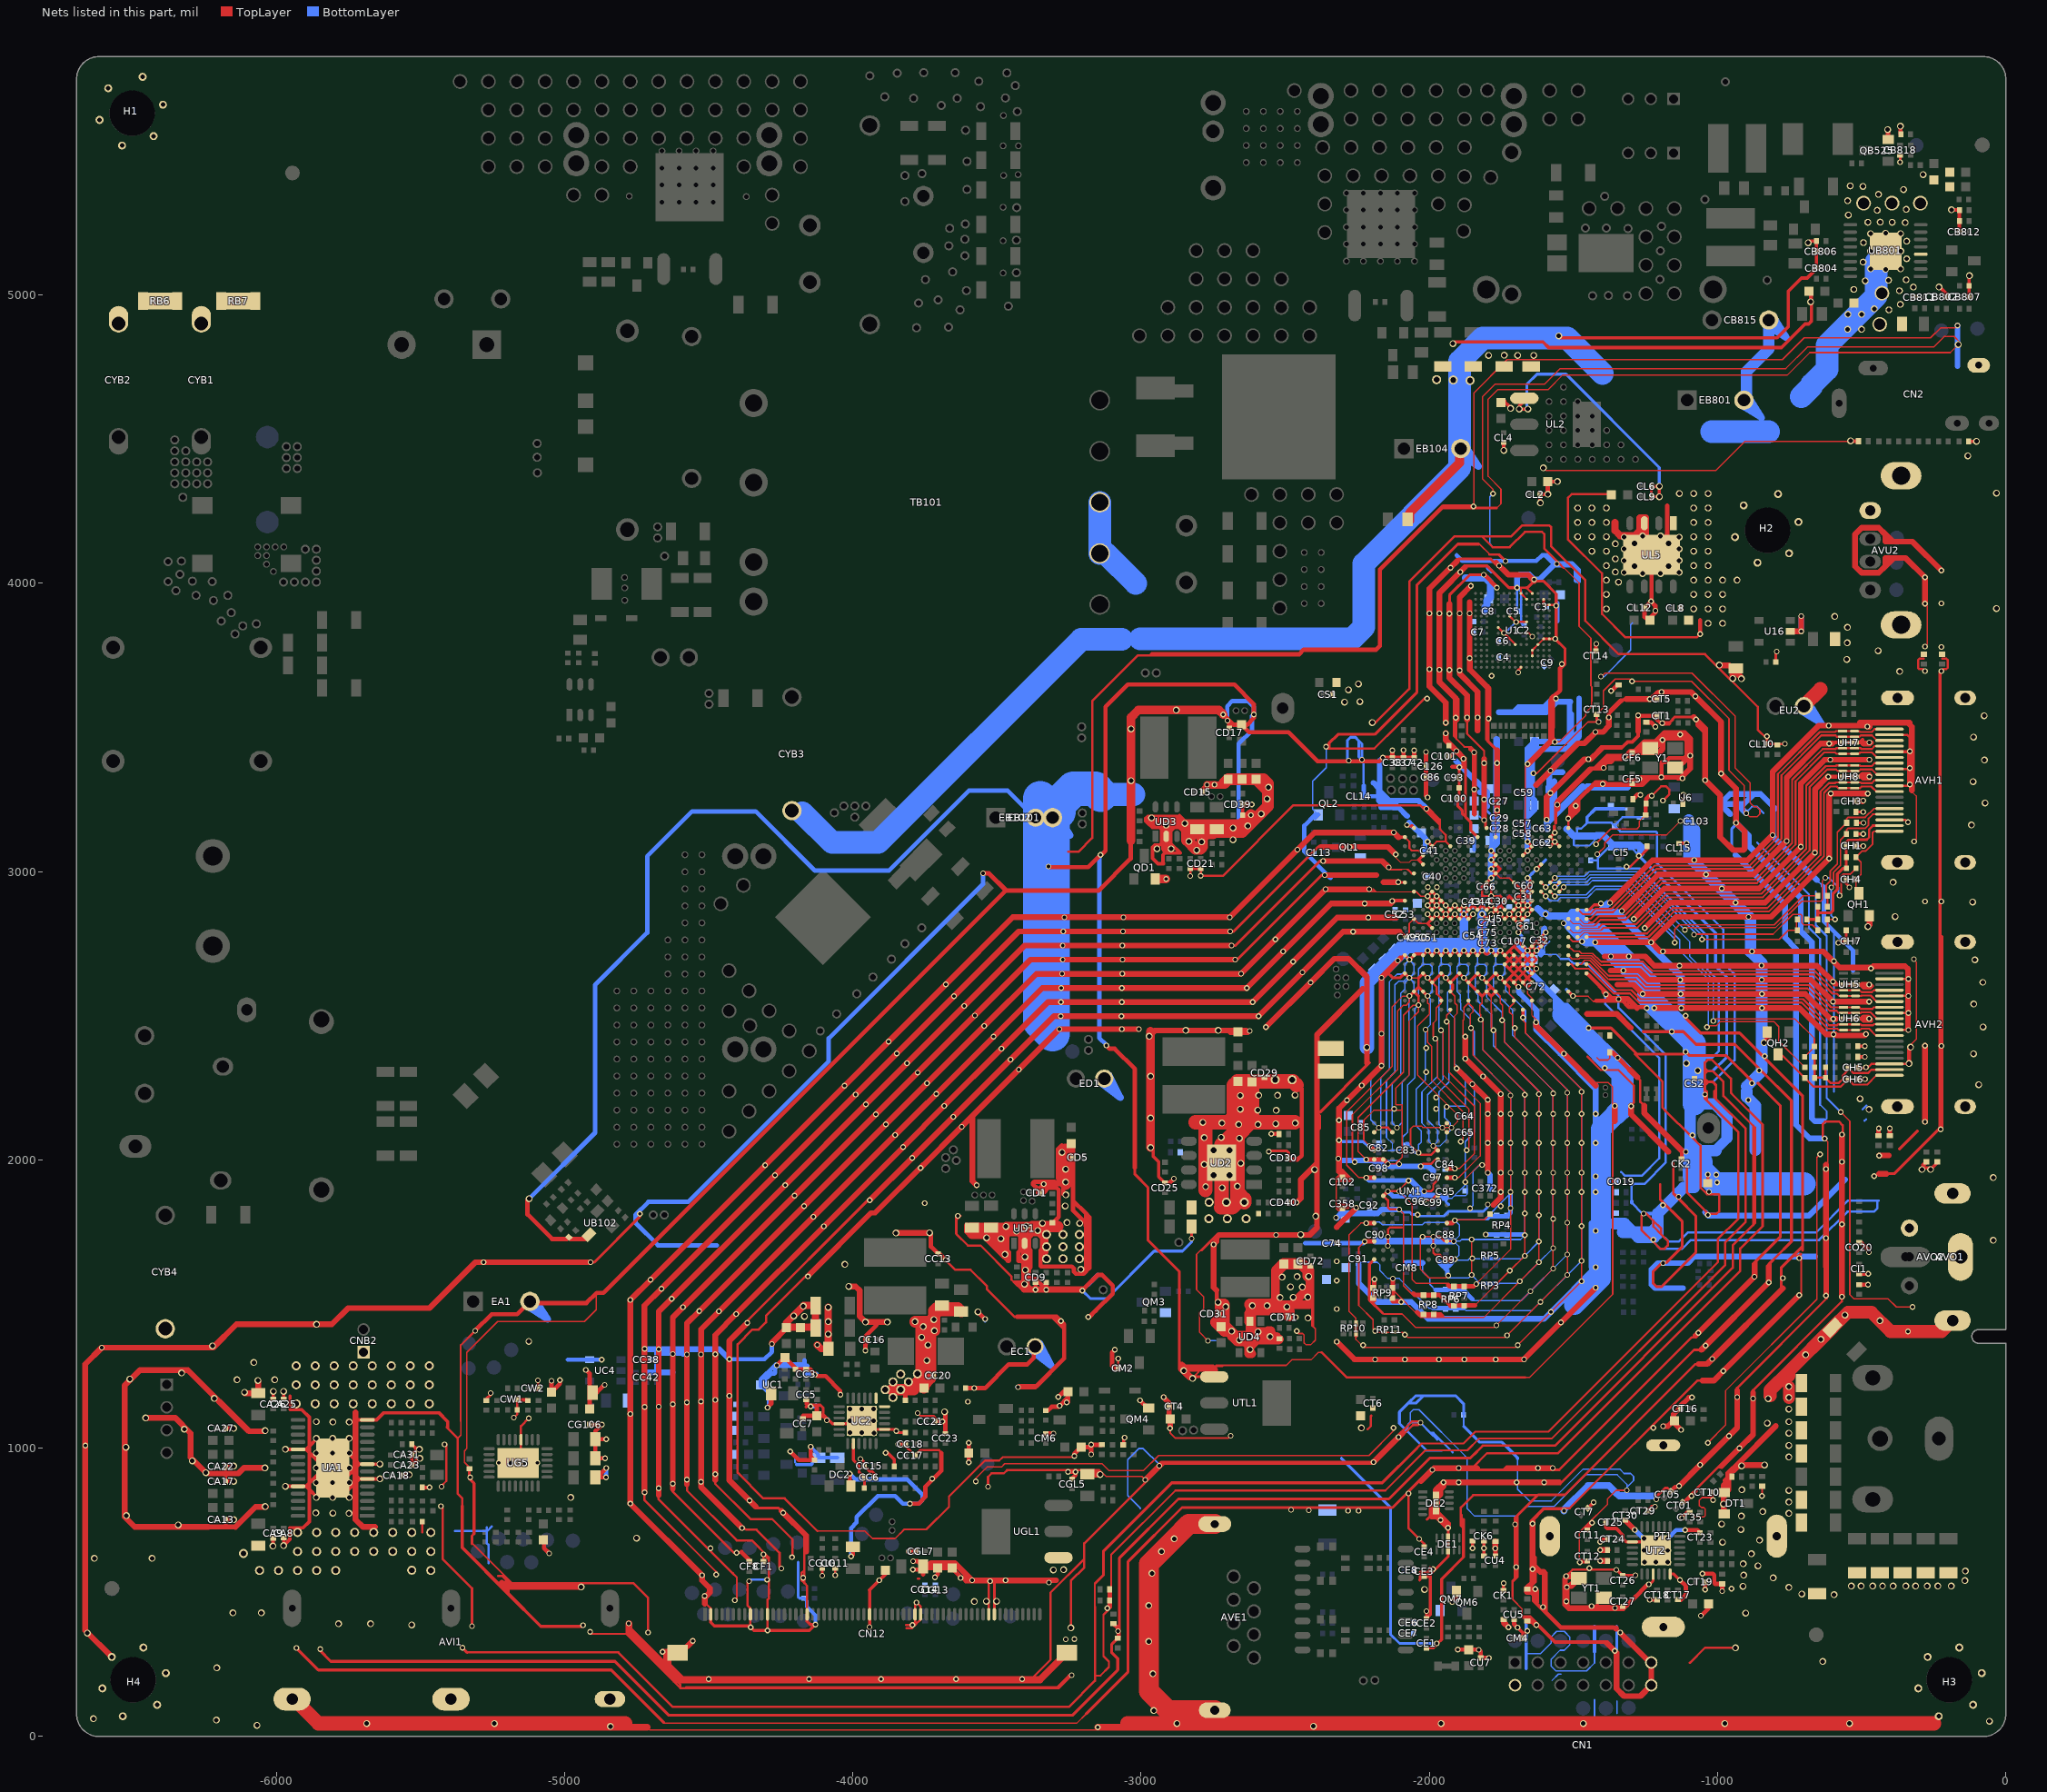
[diagram p0: the nets of this part, all layers, seen from the top]
# Altium PCB MISC84395.PcbDoc (part 19 of 26)
Units mil, origin at the board's own origin, x right, y up, seen from the top; angles counter-clockwise.
Board outline 6692.91 x 5826.77 mil, 2 copper layers (TopLayer, BottomLayer), stack 61.855 mil thick; 951 components, 565 nets, 4374 pads, 1804 vias.
Unrouted connection lines stored in the file: 1.

## Via types
v1: diameter 19.68, hole 11.81, TopLayer to BottomLayer, tented both sides, 1262 vias
v2: diameter 23.62, hole 15.75, TopLayer to BottomLayer, tented both sides, 524 vias
v3: diameter 31.5, hole 19.68, TopLayer to BottomLayer, tented both sides, 11 vias
v4: diameter 24, hole 16, TopLayer to BottomLayer, tented both sides, 6 vias
v5: diameter 19, hole 11.81, TopLayer to BottomLayer, tented both sides, 1 vias

## Nets (pads, with @x,y where several pads share a name; then routed paths per layer and width w, separated by ;. In a path a pad name is that pad's centre, name@x,y a point inside that pad or via, vN(x,y) a via of type N, cw(c..) or ccw(c..) an arc to the next point about the centre after c; other vN are vias at no path point) (continued)
GND: (continued)
  BottomLayer w20: v1@-4722.5,1343 v1(-4673.5,1343) -4463,1343 v1(-4428.5,1308.5) ; CC42.2@-4716,1262.46 RC31.1@-4679,1262.46 ; -4624.46,1262.46 RC31.1@-4679,1262.46 ; -4589,1328 -4591,1330 -4679,1330 RC31.1@-4679,1262.46 ; v1(-1908.55,3533.74) -1908.55,3531.89 v1@-1906.65,3529.99 ; -1906.65,3382.47 -1881.15,3356.97 C26.1@-1799.15,3274.97 ; -1824.78,3274.97 -1806.22,3274.97 C26.1@-1799.15,3274.97 ; -1799.15,3226.74 C26.1@-1799.15,3274.97 ; -1759.65,3552.74 -1707.65,3552.74 ; v1(-1695.65,3984.74) -1695.65,4019.87 -1685.78,4029.74 -1653.65,4029.74 v1(-1636.65,4012.74) -1618.65,4012.74 -1566.35,4065.04 v1@-1564.15,4067.24 ; -1689.7,2743.77 -1683.77,2743.77 -1665.85,2725.85 -1655.42,2715.42 -1655.42,2697.07 -1662.66,2689.82 -1662.66,2664.62 -1608.01,2609.96 -1608.01,2607.83 ; -1653.08,3196.76 -1636.19,3213.65 C55.1@-1636.19,3231 -1636.19,3248.35 -1644.08,3256.24 -1644.08,3405.63 ; v1@-1633.27,510.73 v1(-1633,511) ; v1(-1628.24,2725.85) -1627.69,2725.85 -1616.72,2736.82 ; C72.1@-1621.58,2621.07 -1561.83,2561.32 ; -1613.82,2712.88 -1606.49,2720.21 ; -1603.39,2777.66 -1603.39,2799.74 -1600.39,2802.74 ; v1@-1589.5,3184.5 -1576.82,3197.18 -1576.82,3264.82 -1588,3276 -1588,3292.28 -1583.87,3296.41 ; -1580.65,3591.74 -1602.65,3569.74 -1690.65,3569.74 -1707.65,3552.74 ; -1567,3216 -1567,3313.28 -1583.87,3296.41 ; -1538.01,3344.95 -1571.15,3344.95 -1571.89,3345.69 -1583.87,3345.69 -1583.87,3296.41 ; -1510.65,3588.74 -1558.07,3588.74 -1594.07,3552.74 -1707.65,3552.74 ; -1119.84,1555.16 -1216.48,1555.16 -1228.84,1567.52 -1228.84,1620.16 -1207.2,1641.8 v1(-1189,1641.8) -1103.96,1641.8 -1080.76,1665 -662,1665 ; -1043.29,1818.5 -1031.94,1807.16 -683.22,1807.16 -558.44,1931.94 ; -955.99,3199 -990.99,3234 ; -938.62,3058.12 -766.46,2885.96 -766.46,2770.58 -728,2732.12 -728,2121.5 -680.63,2074.13 v1(-629,2074.13) ; v1(-935.99,3169.07) -891.31,3124.39 -891.31,3088.59 -711.46,2908.74 -711.46,2793.36 -673,2754.91 -673,2144.28 -662.85,2134.13 -631.13,2134.13 ; v1(-900.83,3202) -932.83,3234 ; -799.83,3218 -808.31,3226.47 ; v1@-719.46,1665.47 v1@-716.84,1668.09 ; v1(-709.84,3833) v1(-709.84,3886) ; -655.59,2970.25 -808.31,3122.97 -808.31,3226.47 ; -168,4753 -168,4864 ; v2@-168,4831 -168,4864 ; v1(-168,4894) -168,4864 ; -1561.83,2561.32 -1535.09,2534.57 -1522.81,2534.57 -1446.73,2458.49 -1490.24,2458.49 -1494.67,2458.49 C106.1@-1539.5,2503.33 -1561.83,2525.66 -1561.83,2561.32 ; -990.99,3234 -956.15,3268.84 -874.12,3268.84 ; -990.99,3234 -932.83,3234 ; -932.83,3234 -908.97,3234 -874.12,3268.84 ; -874.12,3268.84 -850.68,3268.84 -808.31,3226.47
  BottomLayer w23.62: EB101.2@-3307.15,3187 -3305.99,3187 -3267,3225.99 ; C90.1@-2187.29,1717.65 -2187.29,1717.97 v1(-1915.64,1717.97)
  BottomLayer w24: v1(-1785.72,2977.82) v1(-1785.72,3009.31) v1(-1785.72,3040.81) -1785.72,3045.21 -1782.21,3048.72 -1782.21,3051.5 -1781.97,3051.74 -1781.97,3084.13 -1766.47,3099.63 -1766.47,3151.31 -1766.47,3458.56 ; v1(-1533,783) -1533,787 -1449,871 -1378.04,871 -1353.02,845.98 -1341.04,834 -1222,834
  BottomLayer w25: -1875.35,4018.03 -1805.34,4018.03 -1788.17,4000.86 -1788.17,3952.03 C108.1@-1794.46,3945.74 -1800.98,3939.22 -1800.98,3923.3 -1807.74,3916.54 C8.1@-1807.74,3902.74 ; -1623.84,2871.76 -1607.82,2855.74 -1597.44,2855.74 -1587.09,2845.4 -1517.69,2845.4 -1503.69,2859.4 -1410.7,2859.4 ; C63.1@-1592.83,3147.83 C63.1@-1590.92,3149.74 -1590.91,3171.47 -1468.65,3293.74 ; -1522.65,3147.74 -1497.65,3122.74 -1487.65,3122.74 -1422.26,3122.74 -1419.31,3125.69 -1396.66,3125.69 -1363.37,3092.4 ; -1451.65,3293.74 -1313.7,3293.74 ; v1@-1381.15,2888.96 -1410.7,2859.4 ; -1353.18,3082.2 -1353.45,3082.47 -1363.37,3092.4 ; -1266.15,3062.36 -1266.15,3086.01 -1272.54,3092.4 -1363.37,3092.4 ; v1(-1125.83,2526.9) -1125.83,2635.24 -1349.99,2859.4 -1410.7,2859.4
  BottomLayer w30: -1880.2,2745.28 v1(-1880.2,2851.83) ; -1824.76,2744.72 -1818.59,2750.9 C75.1@-1818.59,2792.52 ; v1(-1817.21,2851.83) -1818.59,2850.45 -1818.59,2837.74 ; -1798.22,2724.06 -1813.78,2739.62 -1813.78,2787.71 C75.1@-1818.59,2792.52 ; -1634.71,3404.04 C56.1@-1634.71,3451.34 ; C75.1@-1818.59,2792.52 -1818.59,2809.09 ; -1818.59,2809.09 -1818.59,2837.74 ; -1818.59,2809.09 -1808.77,2818.91 -1808.77,2827.92 -1818.59,2837.74
  BottomLayer w34: -1005.86,2031.95 -1005.86,2035.75 -967.92,2073.68 -967.92,2076.65
  BottomLayer w39.37: -1096.03,2023.03 -1096.03,2179.24 -1080.8,2194.47 -1011.88,2194.47 -967.92,2150.51 -967.92,2076.65 ; -1057,2031.95 -1005.86,2031.95 ; EB801.2@-899.5,4644.3 -899.5,4735 -822.57,4811.93 -822.57,4850.5 ; -822.57,4826 -822.57,4850.5 ; CB815.2@-822.57,4912 -822.57,4850.5
  BottomLayer w40: -1359,1779 -1322.96,1779 -1293.11,1749.16 ; -1329.16,1749.16 -1293.11,1749.16 ; -1099.8,3178.58 -1099.8,3156.65 ; -1093.84,3157.16 -1080.32,3143.65 -1080.32,3137.17 ; -1080.8,1943.9 -1080.8,1904 -1118.32,1904 -1208,1814.32 -1208,1786.27 ; v1@-1080.32,3045.67 -1080.32,3137.17 ; -899,2238.1 -899,2218.32 -869,2188.32 -869,2034 ; -899,2255.1 -847.3,2306.79 -847.3,2683.14 -885.46,2721.29 -885.46,2836.67 -1099.8,3051.01 -1099.8,3156.65 ; -1293.11,1749.16 -1275.96,1732 v1@-1223.48,1732 ; -1293.11,1749.16 -1230.57,1749.16 -1208,1771.73 -1208,1786.27 ; v1@-1223.48,1732 -1207.16,1748.32 ; v1@-1223.48,1732 -1220.27,1732 -1207.16,1745.12 -1207.16,1748.32 ; -1208,1786.27 -1207.16,1785.43 -1207.16,1748.32 ; -1099.8,3156.65 -1080.32,3137.17
  BottomLayer w50: v2(-2216.77,2390.46) -2216.77,2614.62 -2216.65,2614.74 -2087.26,2744.12 -2062.3,2744.12 -2061.7,2744.72 -1824.76,2744.72
  BottomLayer w70: -1497,1497 -1404.83,1589.17 -1404.83,1776.93 -1404.83,2107 -1351.83,2160
  BottomLayer w76: C106.1@-1535.33,2506 -1535.33,2503.58 -1490.24,2458.49 -1330.18,2298.42 -1330.18,2181.66 -1351.83,2160
  BottomLayer w78.74: -4175,3204 -4072,3101 -3912,3101 -3208,3805 -3067,3805 ; TB101.9@-3143.53,4280.51 TB101.8@-3143.53,4103.35 -3122.35,4103.35 -3018,3999 ; -3003,3807 -2268,3807 -2227,3848 -2227,4068 -1895.57,4399.43 -1895.57,4446.85 -1895.57,4769.43 -1815,4850 -1615,4850 -1522,4850 -1399.5,4727.5 ; -1020,4526 -823,4526 ; -710,4647 -673.7,4683.3 -673.7,4688.94 -620.87,4741.76 -620.87,4825.41 -450,4996.28 -450,5114
  BottomLayer w80: -3267,3225.99 -3225.99,3267 -3139.72,3267 -3025,3267 ; -1495.52,2824.48 -1451.55,2780.51 -1413.62,2780.51 -1238.8,2605.69 -1238.8,2562.55 -1080.8,2404.55 -1080.8,2194.47 ; -1080.8,2023.03 -1080.8,1943.9 -1075.9,1939 ; -1056.84,1992.41 -1056.84,1966.28 -1008.06,1917.5 -699.5,1917.5
  BottomLayer w120: -3350,3254 -3350,2478.91 -3307.15,2436.06 -3307.15,3164.02 EB101.2@-3307.15,3187 -3287,3207.15 -3287,3234.28 -3234.28,3287 -3159.72,3287 -3139.72,3267
  other v1: -1356.73,296.85 -1828.62,300.62 -5847,303 -3261.5,337 -3231.5,338 -4296,367.66 -1356,446 -1606,449 -4514,488 -3320,534 -4297.18,544 -4172,551 -1351.29,578.23 -1987.32,580.62 -1699,588 -1407,647 -4494,653 -2035.21,685.57 -1436,741 -2282,783 -2246,783 -2418,785 -2480,786 -1090.4,834.5 -1602,882 -3573.71,884.84 -5327,899 -1623.5,931 -5228,949 -5094,949 -5416.23,1013 -960.45,1042.47 -1223,1071 -3601,1161 -4263.22,1287.7 -2188.27,1308.03 -2084.93,1308.03 -1966.82,1308.03 -1878.24,1308.03 -1769.97,1308.03 -1041.72,1355.98 -2230.11,1357.25 -1693.69,1357.25 -340,1405 -2188.27,1406.46 -1543.59,1435.99 -4464.4,1475.03 -2321.15,1482.74 -4588.71,1489.31 -4628.72,1518.59 -624,1529 -2321.15,1581.16 -774,1590 -2321.15,1648.26 -1850.76,1658.41 -717,1659 -1986.51,1702.22 -2143.99,1733.72 -1423.02,1753.92 -1472.23,1770.56 -1521.45,1782.51 -1570.66,1795.33 -2323.62,1799.76 -1619.87,1807.86 -1034,1809 -1669.08,1814.64 -1718.3,1832.36 -2253.99,1833.85 -1752.74,1839.53 -1190,1843 -1797.3,1844.91 -3751,1850 -4201.82,1876.2 -1752.74,1888.74 -1669.08,1888.74 -1619.87,1888.74 -1570.66,1888.74 -1521.44,1888.74 -1472.23,1888.74 -457,1944 -1004.41,1948.42 -1752.74,1955.18 -1718.29,1955.18 -1669.08,1955.18 -1619.87,1955.18 -1570.66,1955.18 -1521.44,1955.18 -1472.23,1955.18 -4304.17,1981.74 -2104.62,1985.69 -1110,2028 -1870.85,2033.92 -1797.03,2058.52 -1752.74,2058.52 -1718.29,2058.52 -1669.08,2058.52 -1619.87,2058.52 -1570.66,2058.52 -1521.44,2058.52 -1472.23,2058.52 -3853.06,2086.36 -3919.97,2158.05 -1797.03,2159.41 -1752.74,2159.41 -1718.29,2159.41 -1669.08,2159.41 -1619.87,2159.41 -1570.66,2159.41 -1521.44,2159.41 -1472.23,2159.41 -2121.84,2176.63 -1976.66,2176.63 -1939.75,2184.01 -2285.86,2207 -894,2208 -1976.66,2216 -1718.3,2223.38 -1669.08,2225.84 -1619.87,2228.31 -3710.48,2228.95 -1570.66,2230.77 -1472.23,2235.69 -2235.03,2257.83 -3775.38,2302.64 -2011.11,2304.58 -1346.8,2354.14 -837.15,2359.99 -2011.11,2388.25 -3512.01,2427.42 -2166.13,2437.46 -1159,2445 -2623,2447 -338.37,2450.71 -1856.09,2457.14 -3576.91,2501.11 -338.37,2509.76 -338.37,2568.82 -1128.65,2575.74 -600,2618 -1129.65,2624.74 -2440.45,2650.55 -1659.73,2662.86 -1132.65,2673.74 -2109.54,2691.39 -319,2696 -2506.97,2722.62 -1189.65,2722.74 -1597,2852 -281,2896 -223.83,2896 -2129.06,2897.57 -2116.65,3059.74 -2123.65,3135.74 -2077.58,3161.48 -1492.65,3227.74 -1272,3322 -333.37,3358.78 -2012,3415 -333.37,3416.78 -1794.65,3530.74 -1560.65,3599.74 -1784,3679 -1692.21,3690.34 -280.83,3695.5 -1540.65,3719.74 -223.83,3779 -1563.62,3807.03 -223.83,3930 -1892.65,4038.74 -1758.33,4061.24 -367,5460
  other v2: -4841,35 -2402,36 -6067,39 -57,53 -6208,57 -6634,62 -2956,90 -2959,218 -6206,238 -636,260 -6655,359 -5530,387 -5784,391 -5673,391 -903,428 -6150,429 -6052,429 -3578.5,468 -3536.5,469.5 -3501.5,469.5 -596,492 -708,494 -2017,510 -753,517 -912,521 -536,522 -502.57,522 -462.57,522 -428,522 -391,522 -347,522 -313,522 -273,522 -236,522 -190,522 -142,541 -807,550 -910,560 -2962,566 -141,574 -3304,578 -3269,579 -860,592 -911,599 -1254.34,604.53 -1213.81,604.28 -1172.92,604.41 -6631,618 -6431,618 -883,634 -1255.16,645.42 -1172.72,645.25 -983,674 -855,681 -1254.99,686.64 -1214.11,686.47 -4750,688 -919,718 -6340,734 -986,737 -918,765 -6520,766 -5747.94,774 -752.76,773.79 -5803.94,775 -5862.94,776 -844,780 -980,806 -752.76,813.79 -5861.24,829.58 -5804.15,829.58 -5747.07,829.58 -4979,829 -752.76,853.79 -916,856 -5861.24,880.76 -5804.15,880.76 -5747.07,880.76 -5861.24,931.94 -5747.07,931.94 -917,939 -5186,949 -5136,949 -6291,956 -5501.56,964.94 -752.76,969.79 -5861.24,983.12 -5804.15,983.12 -5747.07,983.12 -5503.27,996.65 -6521,1003 -752.76,1009.79 -5861.24,1034.3 -5804.15,1034.3 -5747.07,1034.3 -753,1052 -3968.66,1053.73 -3926.59,1053.07 -4009.8,1053.95 -6319,1066 -6148.23,1069 -2236,1070 -828,1087 -5803.94,1091 -5746.94,1091 -5860.94,1092 -753,1092 -4009.93,1094.84 -3927.55,1095 -4009.71,1135.98 -3968.82,1136.11 -3927.68,1135.89 -753,1136 -825,1172 -6214.94,1173 -753,1176 -6109.94,1194 -6063.94,1235 -6135.94,1237 -6004.94,1237 -6508,1240 -2821,1242 -6328,1261 -6077.94,1297 -3743,1304 -694.34,1323.66 -6221,1355 -3739,1358 -5124,1370.5 -2659,1375 -641.98,1377.53 -3761,1385 -2553,1387 -2594,1404 -2686,1406 -3755.57,1421.43 -437.43,1442.43 -3719,1446 -2421,1452 -4168,1457 -4205,1459 -558.35,1461.6 -2494,1490 -2706,1491 -4172,1493 -2614,1494.26 -2563,1494.26 -2733,1506 -2518,1522.26 -2472,1523 -2422,1524.26 -2441,1559 -2482,1560 -2511,1593.26 -2459,1595.26 -2419,1596.26 -3401,1618 -4028,1638 -44,1721 -2446,1741 -3432,1753 -3359,1755 -3469,1769 -3398,1771 -3342,1780 -3213,1780 -3257,1783 -2394,1805 -3263,1840 -3261,1879 -2719,1903 -2776,1907 -2666,1909 -44,1939 -2398,1966 -2781,1984 -2654,1988 -3274,2026 -2659,2075 -2781,2077 -2722,2078 -2661,2123 -2594,2123 -2533,2125 -2720,2128 -2465,2128 -2786,2130 -2531,2172 -2595,2173 -474.55,2175.28 -2656,2176 -506,2211.85 -2656,2223 -2592,2224 -2527,2224 -2466,2225 -94.37,2260.84 -1069,2309.51 -1108,2335 -112.37,2367.84 -79.37,2460.84 -111.37,2540.84 -80.37,2615.84 -107.37,2693.84 -384,2844 -115.37,2894.16 -391.36,2963.29 -2630,3158 -119.37,3161.16 -2583,3200 -72.37,3238.16 -2563,3252 -2558,3292 -114.37,3312.16 -74.37,3387.16 -112.37,3466.16 -75.37,3540.16 -2294,3588 -2241,3589 -2281,3630 -2246,3651 -368.29,3694 -551.83,3736 -443,3766 -550.83,3793 -549.83,3847 -32.5,3912.4 -1260.33,4033.47 -1198.07,4033.47 -1324.58,4037.62 -1133.83,4037.62 -1324.58,4078.24 -1133.83,4078.24 -1324.58,4118.86 -1133.83,4118.86 -1324.58,4159.47 -1133.83,4159.47 -1260.33,4163.62 -1198.08,4163.62 -32.5,4313 -132,4442 -1742,4461 -417.58,5088.39 -469.55,5090.37 -365.61,5090.37 -470.33,5151.39 -364.82,5151.39 -469.55,5212.42 -365.61,5212.42 -417.58,5214.39 -287,5417
  other v3: -2748.56,1946.69 -2693.44,1946.69 -2748.56,2033.31 -2693.44,2033.31 -1288.26,4059.18 -1170.15,4059.18 -1288.27,4137.92 -1170.15,4137.92
  other v5: -1837.35,1569.72
GVOFF: CC6.2 RC6.1 UC2.8 | length 169.9
  TopLayer w10: UC2.8@-3998.27,1016.18 -3998.27,959.21 -3978.59,939.53 -3978.59,917.7 CC6.2@-3959.89,899 ; RC6.1@-3959.73,862 CC6.2@-3959.73,898.84
HDMI1_5V: AVH1.18 CH1.1 RH1.1 RH2.1 RH4.1 RH5.1 RH8.1 | length 594
  TopLayer w6: -546.2,3109.96 -545.7,3110.46
  TopLayer w8: -545.7,3110.46 -507.06,3110.46 -506.87,3110.65 -483.02,3110.65 -474.38,3119.29 -474.38,3146.59 -461.51,3159.45 AVH1.18@-403.84,3159.45
  TopLayer w10: RH2.1@-693.1,2834 RH5.1@-652.57,2834 -652.57,2857 ; RH4.1@-652.57,2878 -652.57,2857 ; -545.7,3109.46 -553.57,3101.6 RH1.1@-553.57,3050 RH8.1@-553.57,3011 -566.06,3011 -584.83,2992.22 -584.83,2937.99 -600.24,2922.58 -600.24,2864.01 -607.26,2857 -652.57,2857
HDMI1_CLKN_IC: AVH1.12 U5.J1 UH8.4 UH8.5 | length 1408.2
  TopLayer w7: U5.J1@-1455.01,2773.09 -1454.67,2773.43 -1239.8,2773.43 -1151.95,2861.28 -822.88,2861.28 -631.33,3052.83 -631.33,3272.66 -608.87,3295.12 -587.37,3295.12 -581.66,3289.41 UH8.4@-565.81,3289.41 UH8.5@-524.87,3289.41 -506.09,3289.41 -500.37,3295.12 -467.12,3295.12 -449.56,3277.56 AVH1.12@-403.84,3277.56
HDMI1_CLKP_IC: AVH1.10 U5.J2 UH8.3 UH8.6 | length 1440.9
  TopLayer w3.94: U5.J2@-1486.5,2773.09 -1478.63,2773.09 -1462.84,2788.88 -1447.64,2788.88 ; -1447.64,2788.84 -1444.19,2788.84
  TopLayer w7: -1445,2786.25 -1444.19,2785.43 -1244.77,2785.43 -1156.92,2873.28 -827.85,2873.28 -643.33,3057.8 -643.33,3277.63 -613.84,3307.12 -592.37,3307.12 -590.4,3309.09 UH8.3@-565.81,3309.09 UH8.6@-524.87,3309.09 -504.34,3309.09 -502.37,3307.12 -465.38,3307.12 -455.57,3316.93 AVH1.10@-403.84,3316.93
HDMI1_DET_IC: RH8.2 U5.R4 | length 1370.6
  TopLayer w5: v1@-1564.97,2946.59 U5.R4@-1549.5,2962.07 ; -1106.03,2805.28 -799.69,2805.28 -707.97,2897 -642.26,2897 -636.21,2903.05 -636.21,2968.63 v1(-626.83,2978)
  TopLayer w6: v1(-576.83,2917) -571.83,2922 -571.83,2984.75 -565.74,2990.84 -540.26,2990.84 RH8.2@-520.1,3011
  BottomLayer w5: v1@-1558.49,2946.11 -1541.17,2963.42 -1454.3,2963.42 -1438.76,2978.96 -1294.39,2978.96 v1(-1113.38,2797.94)
  BottomLayer w6: v1(-626.83,2978) v1@-626.2,2978 ; v1@-623.52,2975.31 v1@-626.2,2978 ; v1(-576.83,2917) -580.4,2920.57 -580.4,2945.17 -613.24,2978 v1@-626.2,2978
  other v1: -1564.97,2946.11
HDMI1_HPD: AVH1.19 CH4.2 QH1.C RH1.2 | length 316.4
  TopLayer w6: QH1.C@-518.33,2925.03 -520.1,2926.8 CH4.2@-520.1,2973 -502.83,2990.27 -502.83,3032.73 RH1.2@-520.1,3050 -499.15,3070.95 -487.48,3070.95 -462.38,3096.06 -462.38,3135.29 -457.9,3139.76 AVH1.19@-403.84,3139.76
HDMI1_HPD_IC: RH2.2 RH3.2 U5.R5 | length 1018.3
  TopLayer w5: U5.R5@-1580.99,2962.07 v1@-1566.36,2976.7 ; v1(-1054.65,2764.74) -786.09,2764.74 -754.83,2796 -726.57,2796 RH2.2@-726.57,2834
  BottomLayer w5: v1@-1561.54,2983.42 -1462.58,2983.42 -1447.04,2998.96 -1274.73,2998.96 -1054.65,2778.88 v1(-1054.65,2764.74)
  other v1: -1565,2978.06
HDMI1_RX0N_IC: AVH1.9 U5.K3 UH8.2 UH8.7 | length 1495.4
  TopLayer w3.94: U5.K3@-1518,2804.59 -1502.38,2788.97 -1474.69,2788.97 -1466.94,2796.71 -1404.8,2796.71 -1402.82,2798.69
  TopLayer w7: -1402.6,2798.47 -1395.73,2805.33 -1278.03,2805.33 -1172.49,2910.87 -843.42,2910.87 -680.93,3073.37 -680.93,3293.2 -619.95,3354.18 -589.37,3354.18 -583.66,3348.46 UH8.2@-565.81,3348.46 UH8.7@-524.87,3348.46 -510.09,3348.46 -504.37,3354.18 -465.07,3354.18 -447.51,3336.61 AVH1.9@-403.84,3336.61
HDMI1_RX0P_IC: AVH1.7 U5.K2 UH8.1 UH8.8 | length 1450
  TopLayer w3.94: U5.K2@-1486.5,2804.59 -1412.74,2804.59 -1410.63,2806.7
  TopLayer w6: -1410.63,2806.7 -1410.5,2806.83
  TopLayer w7: -1410.86,2807.18 -1400.7,2817.33 -1283,2817.33 -1177.46,2922.87 -848.39,2922.87 -692.93,3078.34 -692.93,3298.17 -624.92,3366.18 -590.37,3366.18 -588.4,3368.15 UH8.1@-565.81,3368.15 UH8.8@-524.87,3368.15 -507.34,3368.15 -505.37,3366.18 -465.38,3366.18 -455.57,3375.98 AVH1.7@-403.84,3375.98
HDMI1_RX1N_IC: AVH1.6 U5.L3 UH7.4 UH7.5 | length 1511.2
  TopLayer w3.94: U5.L3@-1518,2836.08 -1502.25,2820.34 -1477.95,2820.34 -1470.08,2812.46 -1427.47,2812.46
  TopLayer w6: -1426.45,2813.48 -1424.52,2815.41
  TopLayer w7: -1424.17,2815.06 -1406.39,2832.83 -1319.83,2832.83 -1192.79,2959.87 -863.72,2959.87 -729.93,3093.67 -729.93,3313.5 -630.19,3413.23 -592.37,3413.23 -587.55,3408.41 UH7.4@-566.32,3408.41 -510.2,3408.41 -505.37,3413.23 -465.07,3413.23 -447.51,3395.67 AVH1.6@-403.84,3395.67
HDMI1_RX1P_IC: AVH1.4 U5.L2 UH7.3 UH7.6 | length 1473.9
  TopLayer w3.94: U5.L2@-1486.5,2836.08 -1479.45,2836.08 -1463.7,2820.34 -1445,2820.34
  TopLayer w7: -1445,2822.93 -1433.26,2822.93 -1411.36,2844.83 -1324.8,2844.83 -1197.76,2971.87 -868.69,2971.87 -741.93,3098.64 -741.93,3318.47 -635.16,3425.23 -591.37,3425.23 -588.51,3428.09 UH7.3@-566.32,3428.09 UH7.6@-525.37,3428.09 -504.23,3428.09 -501.37,3425.23 -465.38,3425.23 -455.57,3435.04 AVH1.4@-403.84,3435.04
HDMI1_RX2N_IC: AVH1.3 U5.L1 UH7.2 UH7.7 | length 1454.7
  TopLayer w7: U5.L1@-1455.01,2836.08 -1441.12,2836.08 -1418.12,2859.08 -1362.87,2859.08 -1213.09,3008.87 -884.02,3008.87 -778.93,3113.96 -778.93,3333.8 -640.43,3472.29 -591.37,3472.29 -586.54,3467.46 -508.2,3467.46 -503.37,3472.29 -465.07,3472.29 -447.51,3454.72 AVH1.3@-403.84,3454.72
HDMI1_RX2P_IC: AVH1.1 U5.M2 UH7.1 UH7.8 | length 1486.4
  TopLayer w5: U5.M2@-1486.5,2867.58 U5.M2@-1482.57,2867.58
  TopLayer w6: U5.M2@-1482.57,2867.58 -1466.82,2851.83 -1447.6,2851.83
  TopLayer w7: -1447.6,2851.83 -1442.34,2851.83 -1423.09,2871.08 -1367.84,2871.08 -1218.06,3020.87 -888.99,3020.87 -790.93,3118.93 -790.93,3338.77 -645.4,3484.29 -592.37,3484.29 -589.51,3487.15 UH7.1@-566.32,3487.15 -509.23,3487.15 -506.37,3484.29 -465.38,3484.29 -455.57,3494.09 AVH1.1@-403.84,3494.09
HDMI1_SCL: AVH1.15 DH2.K RH4.2 RH7.1 | length 500
  TopLayer w6: RH4.2@-619.1,2878 RH7.1@-619.1,2916 -623.52,2920.42 -623.52,2952.6 -608.83,2967.28 -608.83,3002.17 -584.83,3026.17 -584.83,3136.56 DH2.K@-552.61,3168.79 -552.61,3183.06 -547.7,3187.96 -540.88,3187.96 -540.55,3188.29 -532.41,3188.29 -532.08,3187.96 -488.47,3187.96 -457.93,3218.5 AVH1.15@-403.84,3218.5
HDMI1_SCL_IC: RH7.2 U5.P6 | length 1162.4
  TopLayer w5: U5.P6@-1612.49,2930.57 v1@-1596.74,2914.82 ; v1(-1148.65,2753.74) -1148.65,2799.53 -1132.9,2815.28 -803.83,2815.28 -703.11,2916 RH7.2@-652.57,2916
  BottomLayer w4: -1580.75,2898.83 -1555.73,2898.83 -1546.86,2907.71
  BottomLayer w5: v1(-1596.5,2914.58) -1580.75,2898.83 ; -1546.86,2907.71 -1545.17,2909.4 -1451.75,2909.4 -1422.19,2938.96 -1321.35,2938.96 -1148.65,2766.26 v1@-1148.65,2758.74
HDMI1_SDA: AVH1.16 DH3.K RH5.2 RH6.1 | length 595.3
  TopLayer w6: RH6.1@-619.1,2796 RH5.2@-619.1,2834 ; RH5.2@-611.87,2834 RH5.2@-619.1,2834 ; v1(-605.68,2945.21) -597.83,2953.05 -597.83,2997.61 -573.83,3021.61 -573.83,3109.56 DH3.K@-553.11,3130.29 -553.11,3145.06 -548.2,3149.96 -487.97,3149.96 -476.53,3161.4 -476.53,3184.34 -462.06,3198.82 AVH1.16@-403.84,3198.82 ; v1@-604.68,2943.21 v1@-604.18,2943.71 ; v1(-592.83,2834) RH5.2@-619.1,2834
  BottomLayer w6: v1(-605.68,2945.21) -605.68,2846.84 v1(-592.83,2834)
HDMI1_SDA_IC: RH6.2 U5.R6 | length 1150.9
  TopLayer w5: U5.R6@-1608.11,2962.07 U5.R6@-1612.49,2962.07 v1(-1596.5,2946.08) ; v1(-1081.83,2781) -1079.83,2783 -807.83,2783 -739.48,2851.34 -711.6,2851.34 -707.21,2846.95 -707.21,2821.8 -700.41,2815 -671.57,2815 RH6.2@-652.57,2796
  BottomLayer w4: v1@-1595.05,2945.56 -1578.29,2962.32 -1558.12,2962.32 -1547.01,2973.42
  BottomLayer w5: -1547.01,2973.42 -1458.44,2973.42 -1442.9,2988.96 -1278.87,2988.96 -1076.83,2786.92 -1076.83,2786 v1(-1081.83,2781)
HDMI2_5V: AVH2.18 CH5.1 RH10.1 RH11.1 RH14.1 RH15.1 RH18.1 | length 425.4
  TopLayer w8: RH11.1@-664.1,2358.03 RH18.1@-664.1,2321.03 RH10.1@-664.1,2284.03 -662.89,2285.24 RH15.1@-626.36,2285.24 ; RH14.1@-626.36,2321.24 RH15.1@-626.36,2285.24 ; AVH2.18@-403.84,2312.99 -466.6,2312.99 -478.57,2301.03 -528.26,2301.03 CH5.1@-547.1,2319.88 -547.1,2311.3 -565.78,2292.63 -565.78,2280.93 -580.31,2266.4 -607.51,2266.4 RH15.1@-626.36,2285.24
HDMI2_CLKN_IC: AVH2.12 U5.F3 UH6.4 UH6.5 | length 1221.2
  TopLayer w7: U5.F3@-1518,2678.6 -1507.13,2678.6 -1502.09,2673.56 -1502.09,2672.15 -1492.96,2663.02 -1446.83,2663.02 -1361.15,2577.34 -1304.51,2577.34 -1272.56,2545.4 -1041.38,2545.4 -988.91,2545.4 -708.75,2545.4 -618.33,2454.97 -584.37,2454.97 -579.93,2450.54 UH6.4@-562.81,2450.54 -505.81,2450.54 -501.37,2454.97 -474.55,2454.97 -450.68,2431.1 AVH2.12@-403.84,2431.1
HDMI2_CLKP_IC: AVH2.10 U5.F1 UH6.3 UH6.6 | length 1143.4
  TopLayer w7: U5.F1@-1455.01,2678.14 U5.F1@-1455.01,2678.6 -1445.44,2678.6 -1356.18,2589.34 -1299.53,2589.34 -1267.59,2557.4 -1046.35,2557.4 -983.94,2557.4 -703.78,2557.4 -613.36,2466.97 -586.37,2466.97 -583.12,2470.22 UH6.3@-562.81,2470.22 UH6.6@-521.87,2470.22 -503.62,2470.22 -500.37,2466.97 -461.43,2466.97 -457.93,2470.47 AVH2.10@-403.84,2470.47
HDMI2_DET_IC: RH18.2 U5.P5 | length 1333.6
  TopLayer w5: U5.P5@-1580.99,2930.57 v1(-1565,2914.58) ; v1(-1037,2461) -1033.29,2464.71 -1005.18,2464.71 -990.49,2479.4 -804.97,2479.4 -788,2462.43 -788,2411.51 RH18.2@-697.57,2321.03
  BottomLayer w5: v1(-1565,2914.58) -1559.5,2920.08 -1558.82,2919.4 -1455.89,2919.4 -1426.33,2948.96 -1317.2,2948.96 -1131.3,2763.06 -1131.3,2726.01 -1032.51,2627.22 v1@-1032.51,2461
HDMI2_HPD: AVH2.19 CH6.2 QH2.C RH10.2 | length 464.6
  TopLayer w7: QH2.C@-790.5,2366 -779.54,2366 RH10.2@-697.57,2284.03 -667.44,2253.9 -573.08,2253.9 CH6.2@-547.11,2279.87 -528.76,2261.53 -480.77,2261.53 -449,2293.31 AVH2.19@-403.84,2293.31
HDMI2_HPD_IC: RH11.2 RH12.2 U5.P4 | length 1324.5
  TopLayer w5: U5.P4@-1549.5,2930.57 v1(-1533.99,2946.08) ; v1(-1015.15,2482.06) -1007.8,2489.4 -731.95,2489.4 -664.27,2421.72 RH12.2@-664.27,2394.03 -664.27,2391.33 RH11.2@-697.57,2358.03
  BottomLayer w5: v1(-1533.99,2946.08) -1526.65,2953.42 -1450.15,2953.42 -1434.62,2968.96 -1308.92,2968.96 -1096.3,2756.34 -1096.3,2705.16 -1015.17,2624.02 v1(-1015.15,2482.06)
HDMI2_RX0N_IC: AVH2.9 U5.F2 UH6.2 UH6.7 | length 1173.5
  TopLayer w4: U5.F2@-1486.5,2678.6 -1473.51,2678.6 -1460.43,2691.69 -1443.68,2691.69 -1378.34,2626.34 -1374.71,2626.34
  TopLayer w5: U5.F2@-1486.5,2678.6 U5.F2@-1486.43,2678.6
  TopLayer w7: -1374.71,2626.34 -1366.65,2626.34 -1340.86,2626.34 -1284.21,2626.34 -1252.26,2594.4 -1061.68,2594.4 -968.61,2594.4 -688.46,2594.4 -611.34,2517.28 -588.24,2517.28 -580.56,2509.59 UH6.2@-562.81,2509.59 UH6.7@-521.87,2509.59 -503.37,2509.59 -501.09,2511.87 -470.02,2511.87 -448.3,2490.16 AVH2.9@-403.84,2490.16
HDMI2_RX0P_IC: AVH2.7 U5.G3 UH6.1 UH6.8 | length 1197.3
  TopLayer w3.94: U5.G3@-1517.7,2710.4 U5.G3@-1517.4,2710.1
  TopLayer w4: U5.G3@-1517.4,2710.1 U5.G3@-1518,2710.1 -1504.91,2697.01 -1480.75,2697.01 -1478.07,2699.69 -1440.37,2699.69 -1379.02,2638.34 -1376.21,2638.34
  TopLayer w5: U5.G3@-1518,2710.1 U5.G3@-1517.7,2710.4
  TopLayer w7: -1376.21,2638.34 -1279.24,2638.34 -1247.29,2606.4 -1066.65,2606.4 -963.64,2606.4 -683.49,2606.4 -606.37,2529.28 UH6.1@-562.81,2529.28 -508.24,2529.28 -502.84,2523.87 -463.58,2523.87 -457.93,2529.53 AVH2.7@-403.84,2529.53
HDMI2_RX1N_IC: AVH2.6 U5.G2 UH5.4 UH5.5 | length 1150.3
  TopLayer w4: U5.G2@-1486.5,2710.1 -1484.09,2707.69 -1437.05,2707.69 -1404.71,2675.34 -1397.21,2675.34
  TopLayer w7: -1397.21,2675.34 -1317.65,2675.34 -1263.91,2675.34 -1231.97,2643.4 -668.16,2643.4 -601.1,2576.33 -586.37,2576.33 -578.69,2568.65 UH5.4@-562.81,2568.65 UH5.5@-521.87,2568.65 -502.01,2568.65 -500.78,2569.87 -468.96,2569.87 -448.3,2549.21 AVH2.6@-403.84,2549.21
HDMI2_RX1P_IC: AVH2.4 U5.H3 UH5.3 UH5.6 | length 1180
  TopLayer w3.94: U5.H3@-1518,2741.6 U5.H3@-1517.39,2741.6
  TopLayer w4: U5.H3@-1518,2741.6 -1517.38,2741.6 -1498.98,2723.19 -1479.71,2723.19 -1472.21,2715.69 -1433.74,2715.69 -1406.55,2688.5
  TopLayer w7: -1403.27,2687.34 -1258.94,2687.34 -1227,2655.4 -663.19,2655.4 -596.13,2588.33 -507.24,2588.33 -500.78,2581.87 -464.64,2581.87 -457.93,2588.58 AVH2.4@-403.84,2588.58